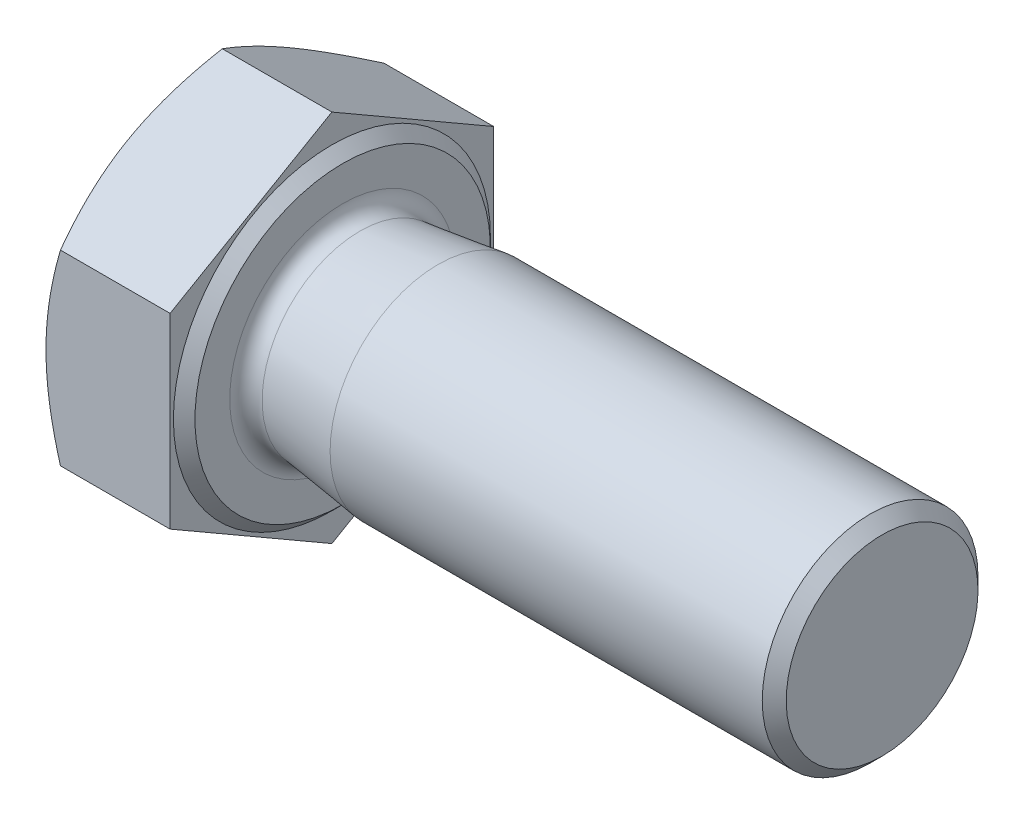
SolidWorks part; units mm, degrees
ref_plane "前视基准面" through (0, 0, 0) normal (0, 0, 1) x (1, 0, 0)
ref_plane "上视基准面" through (0, 0, 0) normal (0, 1, 0) x (1, 0, 0)
ref_plane "右视基准面" through (0, 0, 0) normal (1, 0, 0) x (0, 0, -1)
sketch "草图1" plane through (0, 0, 0) normal (0, 0, 1) x (1, 0, 0)
  line L0 (0, 0) -> (37.5, 0) construction
  line L1 (0, 0) -> (0, 10.015)
  line L2 (0, 10.015) -> (7.5, 10.015)
  line L3 (7.5, 10.015) -> (7.5, 0)
  line L4 (7.5, 6) -> (37.5, 6)
  line L5 (37.5, 6) -> (37.5, 0)
  line L6 (0, 9) -> (0.586, 10.015)
  line L7 (34, 6) -> (34, 0)
  line L8 (12.8, 6) -> (12.8, 0)
  line L9 (7.5, 5.4317) -> (37.5, 5.4317)
  line L10 (37.5, 5.0528) -> (7.5, 5.0528)
  line L11 (6.9, 8.815) -> (7.5, 8.215)
  line L12 (6.9, 10.015) -> (6.9, 0)
  line L13 (7.4, 8.315) -> (7.4, 0) construction
  arc A0 (7.5, 6.85) -> (8.35, 6) centre (8.35, 6.85) ccw
  point P12 (35.75, 0)
  point P13 (2.38, 10.015)
  point P14 (7.5, 6.85)
  point P24 (7.5, 8.315)
  dimension "D1" = 0.1
  dimension "r" = 0.85
  dimension "k" = 7.5
  dimension "D2" = 45
  dimension "β" = 30
  dimension "e" = 20.03
  dimension "s" = 18
  dimension "d" = 12
  dimension "l" = 30
  dimension "D52" = 3.5
  dimension "P" = 1.75
  dimension "kw" = 5.12
  dimension "da" = 13.7
  dimension "a" = 5.3
  dimension "ds" = 10.8634
  dimension "D61" = 10.1056
  dimension "dw" = 16.63
  dimension "c" = 0.6
sketch "草图2" plane through (0, 0, 0) normal (1, 0, 0) x (0, 0, -1)
  line L1 (0, 10.3923) -> (-9, 5.1962)
  line L2 (-9, 5.1962) -> (-9, -5.1962)
  line L3 (-9, -5.1962) -> (0, -10.3923)
  line L4 (0, -10.3923) -> (9, -5.1962)
  line L5 (9, -5.1962) -> (9, 5.1962)
  line L6 (9, 5.1962) -> (0, 10.3923)
  circle A0 centre (0, 0) radius 9 construction
sketch "草图3" plane through (0, 0, 0) normal (1, 0, 0) x (0, 0, -1)
  line L0 (9, 5.1962) -> (0, 10.3923) construction
  line L1 (0, 10.3923) -> (-9, 5.1962) construction
  line L2 (-9, 5.1962) -> (-9, -5.1962) construction
  line L3 (9, -5.1962) -> (9, 5.1962) construction
  line L4 (0, -10.3923) -> (9, -5.1962) construction
  line L5 (-9, -5.1962) -> (0, -10.3923) construction
  line L6 (9, 5.1962) -> (0, 10.3923)
  line L7 (0, 10.3923) -> (-9, 5.1962)
  line L8 (-9, 5.1962) -> (-9, -5.1962)
  line L9 (9, -5.1962) -> (9, 5.1962)
  line L10 (0, -10.3923) -> (9, -5.1962)
  line L11 (-9, -5.1962) -> (0, -10.3923)
extrude "凸台-拉伸1" add sketch "草图3" along normal up to vertex (7.5 mm away) up to point (7.5, 10.015, 0)
sketch "草图4" plane through (0, 0, 0) normal (-1, 0, 0) x (0, 0, 1)
  circle A0 centre (0, 0) radius 9 construction
  circle A1 centre (0, 0) radius 9
  circle A2 centre (0, 0) radius 20.03
  dimension "D1" = 40.06
extrude "切除-拉伸1" cut sketch "草图4" against normal blind 0.9375 draft 60
sketch "草图5" [suppressed] plane through (0, 0, 0) normal (0, 0, 1) x (1, 0, 0)
  line L0 (33, 26) -> (233, 26) construction
  line L1 (233, 26) -> (233, 0) construction
  line L2 (0, 0) -> (233, 0) construction
  line L3 (35.3, 26) -> (233, 26)
  line L4 (233, 26) -> (233, 0)
  line L5 (33, 0) -> (233, 0)
  line L6 (33, 28.3) -> (33, 0)
  arc A0 (33, 28.3) -> (35.3, 26) centre (35.3, 28.3) ccw construction
  arc A1 (33, 28.3) -> (35.3, 26) centre (35.3, 28.3) ccw
revolve "旋转1" add sketch "草图5" angle 360 about L5
cosmetic thread "装饰螺纹线2" [suppressed] parameters "D1"=34.7, "D2"=10.1056
chamfer "倒角2" [suppressed] distance 0.6667 angle 45
sketch "草图7" [suppressed] plane through (0, 0, 0) normal (0, 0, 1) x (1, 0, 0)
  line L0 (33, 37) -> (32, 38)
  line L1 (32, 38) -> (32, 88.25)
  line L2 (32, 88.25) -> (33, 88.25)
  line L3 (33, 88.25) -> (33, 37)
  line L4 (0, 0) -> (233, 0) construction
  line L5 (0, 0) -> (233, 0) construction
  dimension "D1" = 40.06
revolve "切除-旋转1" [suppressed] cut sketch "草图7" angle 360 mid plane about L5
sketch "草图6" plane through (0, 0, 0) normal (0, 0, 1) x (1, 0, 0)
  line L0 (12.8, 0) -> (12.8, 6) construction
  line L1 (12.8, 6) -> (37.5, 6)
  line L2 (37.5, 6) -> (37.5, 0)
  line L3 (12.8, 6) -> (8.459, 5.4387)
  line L5 (7.5, 5.4317) -> (37.5, 5.4317) construction
  line L6 (7.5, 10.015) -> (7.5, 0) construction
  line L7 (7.5, 6.2817) -> (7.5, 0)
  line L8 (7.5, 0) -> (37.5, 0)
  arc A0 (8.459, 5.4387) -> (7.5, 6.2817) centre (8.35, 6.2817) cw
  arc A1 (7.5, 6.85) -> (8.35, 6) centre (8.35, 6.85) ccw construction
revolve "旋转2" add sketch "草图6" angle 360 about L8
cosmetic thread "装饰螺纹线1" parameters "D1"=34.7, "D2"=10.1056
chamfer "倒角1" distance 0.6667 angle 45 1 edges at (37.5, -6, 0)
sketch "草图8" plane through (0, 0, 0) normal (0, 0, 1) x (1, 0, 0)
  line L0 (7.5, 8.215) -> (6.9, 8.815)
  line L1 (6.9, 8.815) -> (6.9, 20.03)
  line L2 (6.9, 20.03) -> (7.5, 20.03)
  line L3 (7.5, 20.03) -> (7.5, 8.215)
  line L4 (0, 0) -> (37.5, 0) construction
  line L5 (0, 0) -> (37.5, 0) construction
  dimension "D1" = 40.06
revolve "切除-旋转2" cut sketch "草图8" angle 360 mid plane about L5
